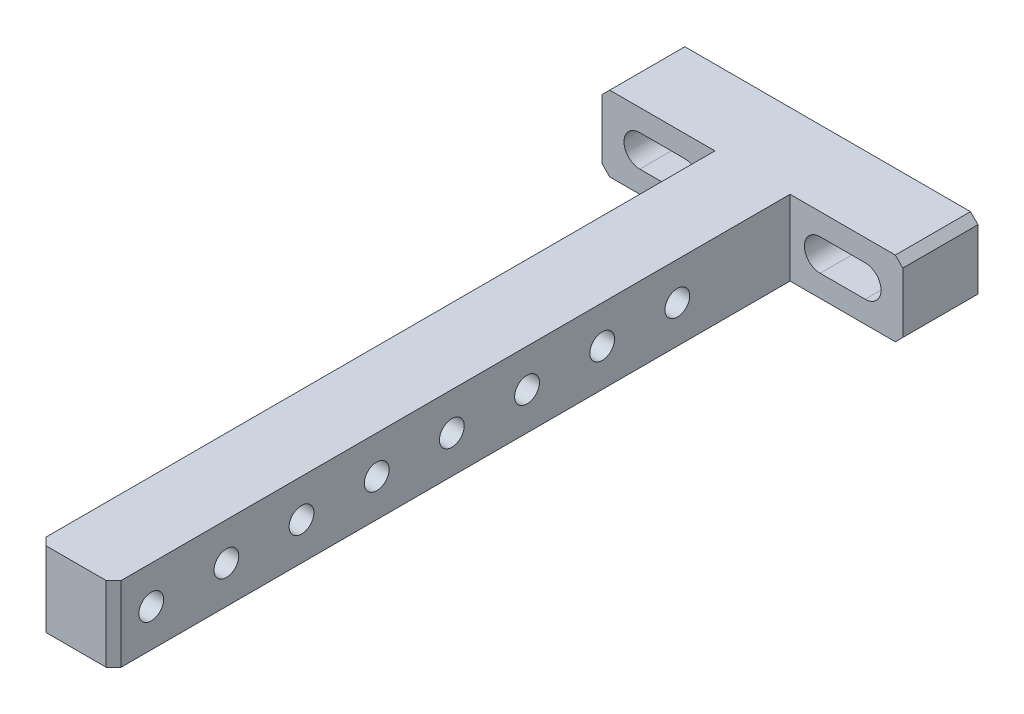
SolidWorks part; units mm, degrees
material "S45C"
ref_plane "Front Plane" through (0, 0, 0) normal (0, 0, 1) x (1, 0, 0)
ref_plane "Top Plane" through (0, 0, 0) normal (0, 1, 0) x (1, 0, 0)
ref_plane "Right Plane" through (0, 0, 0) normal (1, 0, 0) x (0, 0, -1)
sketch "Sketch1" plane through (0, 0, 0) normal (0, 0, 1) x (1, 0, 0)
  line L1 (-20, 5) -> (20, 5)
  line L2 (-20, 5) -> (-20, -5)
  line L3 (-20, -5) -> (20, -5)
  line L4 (20, 5) -> (20, -5)
  line L5 (-20, 5) -> (20, -5) construction
  line L6 (-20, -5) -> (20, 5) construction
  point P0 (0, 0)
  dimension "D1" = 10
  dimension "D2" = 40
extrude "Boss-Extrude1" add sketch "Sketch1" along normal blind 10
sketch "Sketch2" plane through (0, 0, 10) normal (0, 0, 1) x (1, 0, 0)
  line L0 (20, 5) -> (-20, 5) construction
  line L1 (-5, -5) -> (5, -5)
  line L2 (-5, -5) -> (-5, 5)
  line L3 (-5, 5) -> (5, 5)
  line L4 (5, -5) -> (5, 5)
  line L5 (-5, -5) -> (5, 5) construction
  line L6 (-5, 5) -> (5, -5) construction
  point P0 (0, 0)
  dimension "D1" = 10
extrude "Boss-Extrude2" add sketch "Sketch2" along normal blind 90
sketch "Sketch3" plane through (0, 0, 0) normal (0, 0, -1) x (-1, 0, 0)
  line L0 (-15, 0) -> (-9, 0) construction
  line L1 (-15, 2.1) -> (-9, 2.1)
  line L2 (-15, -2.1) -> (-9, -2.1)
  line L3 (0, 5) -> (0, -5) construction
  line L4 (-20, 5) -> (20, 5) construction
  line L5 (20, -5) -> (-20, -5) construction
  line L6 (15, 0) -> (9, 0) construction
  line L7 (15, 2.1) -> (9, 2.1)
  line L8 (15, -2.1) -> (9, -2.1)
  arc A0 (-15, 2.1) -> (-15, -2.1) centre (-15, 0) ccw
  arc A1 (-9, -2.1) -> (-9, 2.1) centre (-9, 0) ccw
  arc A2 (15, 2.1) -> (15, -2.1) centre (15, 0) cw
  arc A3 (9, -2.1) -> (9, 2.1) centre (9, 0) cw
  point P2 (-12, 0)
  point P15 (12, 0)
  dimension "D3" = 2.1
  dimension "D1" = 24
  dimension "D2" = 6
extrude "Cut-Extrude1" cut sketch "Sketch3" against normal through all
sketch "Sketch4" plane through (0, -5, 0) normal (0, -1, 0) x (1, 0, 0)
  line L0 (0, 90) -> (0, 20) construction
  line L1 (2.25, 90) -> (2.25, 20)
  line L2 (-2.25, 90) -> (-2.25, 20)
  line L4 (-20, 0) -> (20, 0) construction
  arc A0 (2.25, 90) -> (-2.25, 90) centre (0, 90) ccw
  arc A1 (-2.25, 20) -> (2.25, 20) centre (0, 20) ccw
  point P3 (0, 55)
  dimension "D1" = 2.25
  dimension "D3" = 70
  dimension "D2" = 20
extrude "Cut-Extrude2" [suppressed] cut sketch "Sketch4" against normal through all
hole_wizard "M4 Tapped Hole1" positions "Sketch6" profile "Sketch7" tap size "M4" standard "Gb" end condition through all
sketch "Sketch6" plane through (5, 0, 0) normal (1, 0, 0) x (0, 0, -1)
  line L0 (-100, -5) -> (-100, 5) construction
  line L1 (-95, 0) -> (-100, 0) construction
  point P2 (-25, 0)
  point P4 (-35, 0)
  point P6 (-45, 0)
  point P8 (-55, 0)
  point P10 (-65, 0)
  point P12 (-75, 0)
  point P14 (-85, 0)
  point P16 (-95, 0)
  dimension "D2" = 10
  dimension "D3" = 10
  dimension "D4" = 10
  dimension "D5" = 10
  dimension "D6" = 10
  dimension "D7" = 10
  dimension "D8" = 10
  dimension "D9" = 5
sketch "Sketch7" plane through (5, 0, 25) normal (0, 1, 0) x (0, 0, -1)
  line L0 (0, 0) -> (0, 25)
  line L1 (0, 25) -> (1.65, 25)
  line L2 (1.65, 25) -> (1.65, 0)
  line L5 (1.65, 0) -> (0, 0)
  line L11 (0, -6.35) -> (0, 107.95) construction
  dimension "通孔螺纹孔钻头直径" = 3.3
  dimension "通孔螺纹孔钻头深度" = 25
cosmetic thread "Cosmetic Thread 1" parameters "D2"=4
cosmetic thread "Cosmetic Thread 2" parameters "D2"=4
cosmetic thread "Cosmetic Thread 3" parameters "D2"=4
cosmetic thread "Cosmetic Thread 4" parameters "D2"=4
cosmetic thread "Cosmetic Thread 5" parameters "D2"=4
cosmetic thread "Cosmetic Thread 6" parameters "D2"=4
cosmetic thread "Cosmetic Thread 7" parameters "D2"=4
cosmetic thread "Cosmetic Thread 8" parameters "D2"=4
chamfer "Chamfer1" distance 1 angle 45 6 edges at (20, 5, 5) (20, -5, 5) (-20, -5, 5) (-20, 5, 5) (5, 0, 100) (-5, 0, 100)
